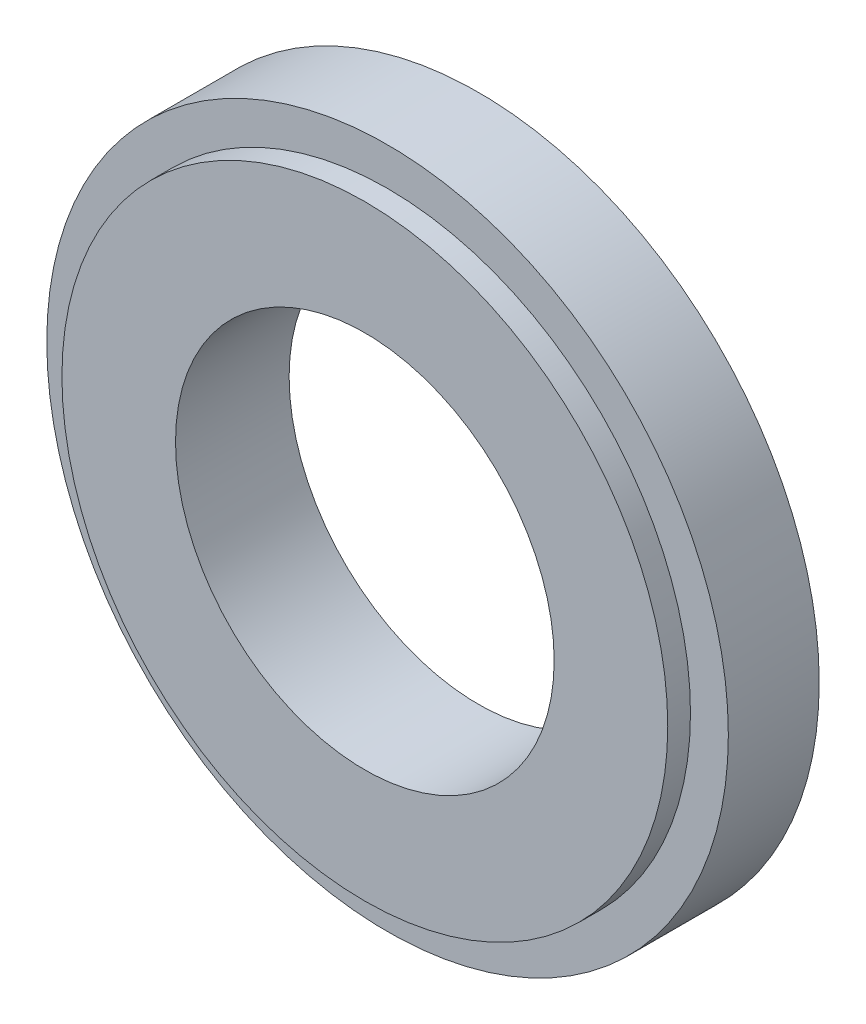
from build123d import *

# Parameters (mm, degrees)
SKETCH1_R             = 45
SKETCH1_R_2           = 25
BOSS_EXTRUDE1_DEPTH   = 12
SKETCH2_R             = 40
SKETCH2_R_2           = 25
BOSS_EXTRUDE2_DEPTH   = 3
M4_TAPPED_HOLE2_D     = 3.3
M4_TAPPED_HOLE2_DEPTH = 10.1
M4_TAPPED_HOLE2_TIP   = 0.991420021


with BuildPart() as part:
    # Sketch1 → Boss-Extrude1 (new body)
    with BuildSketch(Plane.XY):
        Circle(SKETCH1_R)
        Circle(SKETCH1_R_2, mode=Mode.SUBTRACT)
    extrude(amount=BOSS_EXTRUDE1_DEPTH)

    # Sketch2 → Boss-Extrude2 (add)
    with BuildSketch(Plane.XY.offset(12)):
        Circle(SKETCH2_R)
        Circle(SKETCH2_R_2, mode=Mode.SUBTRACT)
    extrude(amount=BOSS_EXTRUDE2_DEPTH)

    # M4 Tapped Hole2
    with Locations(Plane(origin=(32.04293994, 18.5, 0), x_dir=(-1, 0, 0), z_dir=(0, 0, -1))):
        with Locations((0, 0), (32.04293994, 18.5), (64.08587988, 0), (64.08587988, -37), (32.04293994, -55.5), (0, -37)):
            Hole(M4_TAPPED_HOLE2_D / 2, depth=M4_TAPPED_HOLE2_DEPTH)
            with Locations((0, 0, -(M4_TAPPED_HOLE2_DEPTH + M4_TAPPED_HOLE2_TIP / 2))):  # 118° drill point
                Cone(0, M4_TAPPED_HOLE2_D / 2, M4_TAPPED_HOLE2_TIP, mode=Mode.SUBTRACT)


solid = part.part
